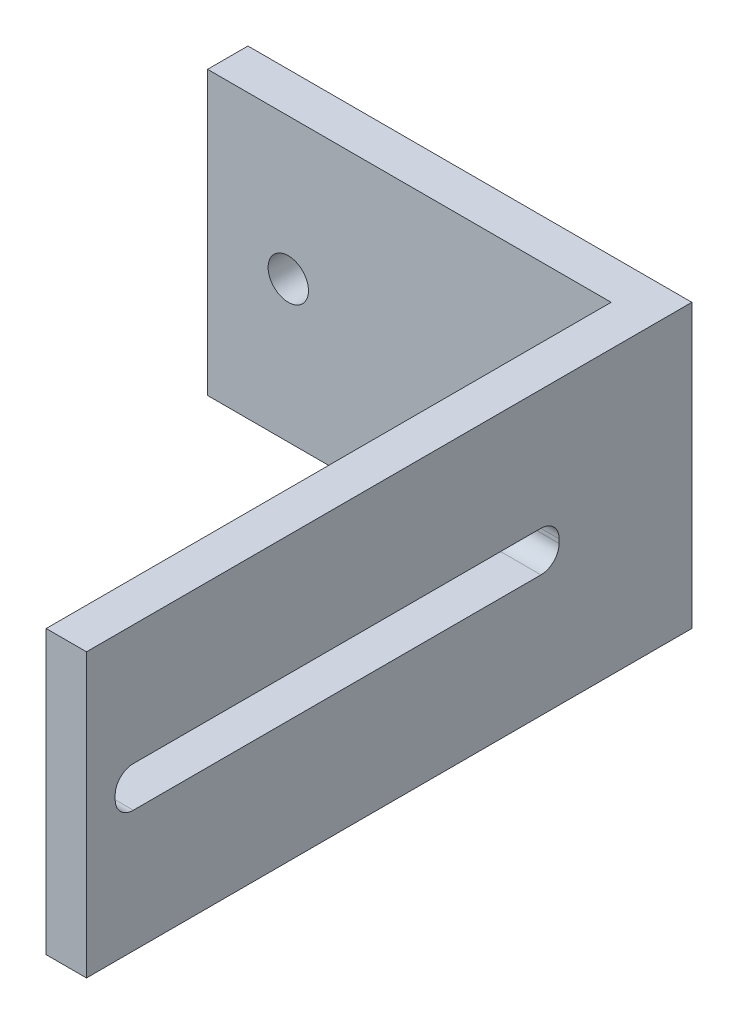
from build123d import *

# Parameters (mm, degrees)
SKETCH1_W           = 100
SKETCH1_H           = 70
BOSS_EXTRUDE1_DEPTH = 10
SKETCH2_R           = 5
CUT_EXTRUDE1_DEPTH  = 10
SKETCH3_W           = 150
SKETCH3_H           = 70
BOSS_EXTRUDE2_DEPTH = 10
CUT_EXTRUDE2_DEPTH  = 50


with BuildPart() as part:
    # Sketch1 → Boss-Extrude1 (new body)
    with BuildSketch(Plane.XY):
        Rectangle(SKETCH1_W, SKETCH1_H)
    extrude(amount=BOSS_EXTRUDE1_DEPTH)

    # Sketch2 → Cut-Extrude1 (cut)
    with BuildSketch(Plane.XY.offset(10)):
        with Locations((-30, 0)):
            Circle(SKETCH2_R)
        with Locations((30, 0)):
            Circle(SKETCH2_R)
    extrude(amount=-CUT_EXTRUDE1_DEPTH, mode=Mode.SUBTRACT)

    # Sketch3 → Boss-Extrude2 (add)
    with BuildSketch(Plane(origin=(50, 0, 0), x_dir=(0, 0, -1), z_dir=(1, 0, 0))):
        with Locations((-75, 0)):
            Rectangle(SKETCH3_W, SKETCH3_H)
    extrude(amount=BOSS_EXTRUDE2_DEPTH)

    # Sketch7 → Cut-Extrude2 (cut)
    with BuildSketch(Plane.ZY.offset(-50)):
        with BuildLine():
            Line((138.396107193, -4.795166993), (37.396107193, -4.795166993))
            ThreePointArc((37.396107193, -4.795166993), (34.214126678, -3.477147509), (32.896107193, -0.295166993))
            Line((32.896107193, -0.295166993), (32.896107193, 0.704833007))
            ThreePointArc((32.896107193, 0.704833007), (34.214126678, 3.886813522), (37.396107193, 5.204833007))
            Line((37.396107193, 5.204833007), (138.396107193, 5.204833007))
            ThreePointArc((138.396107193, 5.204833007), (141.578087709, 3.886813522), (142.896107193, 0.704833007))
            Line((142.896107193, 0.704833007), (142.896107193, -0.295166993))
            ThreePointArc((142.896107193, -0.295166993), (141.578087709, -3.477147509), (138.396107193, -4.795166993))
        make_face()
    extrude(amount=-CUT_EXTRUDE2_DEPTH, mode=Mode.SUBTRACT)


solid = part.part
